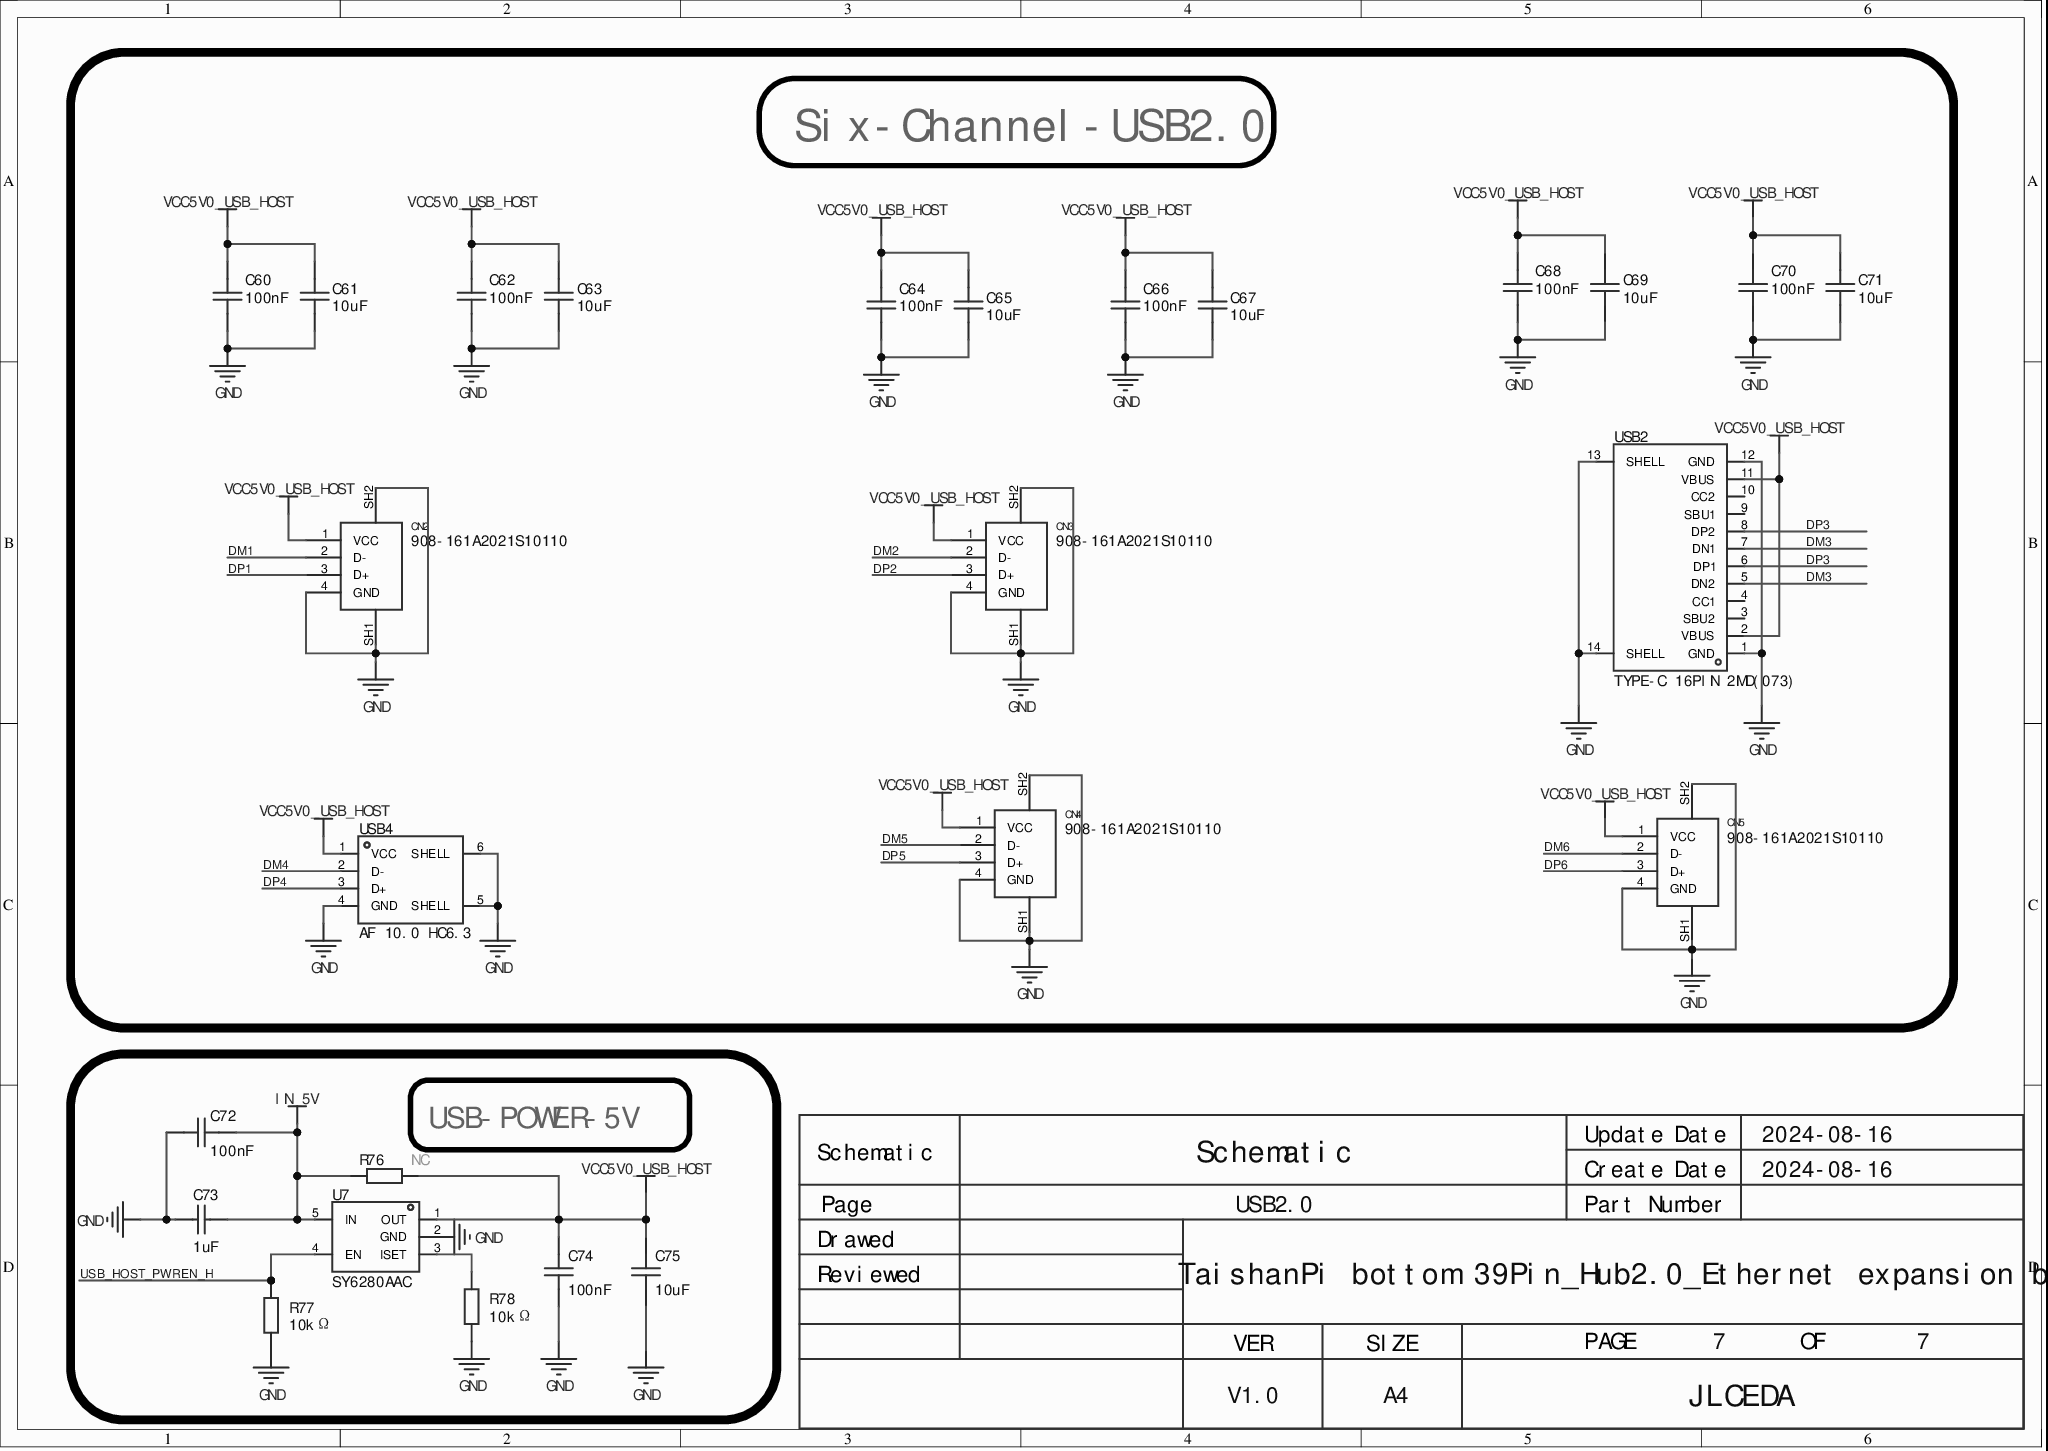
[diagram p0: MISC84334-8.SchDoc]
# Altium project MISC84334.PrjPcb (part 5 of 5)

## Sheet MISC84334-8.SchDoc
size 297 x 210 mm; Symbol: Sheet-Symbol_A4; Company: JLCEDA; Version: V1.0; Page Size: A4; @Project Name: COMPANY_A TaishanPi bottom 39Pin_Hub2.0_Ethernet expansion board; @Page Count: 7; @Update Date: 2024-08-16; @Create Date: 2024-08-16; @Schematic Name: Schematic; @Page No: 7; @Page Name: USB2.0; Device: Sheet-Symbol_A4

### Parts
C60  100nF  [R0402]
C61  10uF  [R0402]
C62  100nF  [r0603]
C63  10uF  [r0603]
C64  100nF  [r0603]
C65  10uF  [r0603]
C66  100nF  [r0603]
C67  10uF  [r0603]
C68  100nF  [r0603]
C69  10uF  [r0603]
C70  100nF  [r0603]
C71  10uF  [r0603]
C72  100nF  [C0603]
C73  1uF  [C0603]
C74  100nF  [C0603]
C75  10uF  [C0603]
CN2  908-161A2021S10110  [USB-A-SMD_AF-SMT-SHORT]
CN3  908-161A2021S10110  [USB-A-SMD_AF-SMT-SHORT]
CN4  908-161A2021S10110  [USB-A-SMD_AF-SMT-SHORT]
CN5  908-161A2021S10110  [USB-A-SMD_AF-SMT-SHORT]
R76  NC  [R0805]
R77  10kΩ  [R0402]
R78  10kΩ  [R0402]
U7  SY6280AAC  [SOT-23-5_L3.0-W1.7-P0.95-LS2.8-BL]
USB2  TYPE-C 16PIN 2MD(073)  [USB-C-SMD_TYPE-C-6PIN-2MD-073]
USB4  AF 10.0 HC6.3  [USB-A-TH_AF-10.0-HC6.3]

### Blocks framed on the sheet
Six-Channel-USB2.0: C60-C71 CN2-CN5 USB2 USB4
USB-POWER-5V: C72-C75 R76-R78 U7

### Nets
GND: C60.1 C61.1 C62.1 C63.1 C64.1 C65.1 C66.1 C67.1 C68.1 C69.1 C70.1 C71.1 C72.2 C73.1 C74.1 C75.1 CN2.4(GND) CN2.SH1 CN2.SH2 CN3.4(GND) CN3.SH1 CN3.SH2 CN4.4(GND) CN4.SH1 CN4.SH2 CN5.4(GND) CN5.SH1 CN5.SH2 R77.1 R78.1 U7.2(GND) USB2.1(GND) USB2.12(GND) USB2.13(SHELL) USB2.14(SHELL) USB4.4(GND) USB4.5(SHELL) USB4.6(SHELL)
IN_5V: C72.1 C73.2 R76.1 U7.5(IN)
VCC5V0_USB_HOST: C60.2 C61.2 C62.2 C63.2 C64.2 C65.2 C66.2 C67.2 C68.2 C69.2 C70.2 C71.2 C74.2 C75.2 CN2.1(VCC) CN3.1(VCC) CN4.1(VCC) CN5.1(VCC) R76.2 U7.1(OUT) USB2.2(VBUS) USB2.11(VBUS) USB4.1(VCC)
DM1: CN2.2(D-)
DM2: CN3.2(D-)
DM3: USB2.5(DN2) USB2.7(DN1)
DM4: USB4.2(D-)
DM5: CN4.2(D-)
DM6: CN5.2(D-)
DP1: CN2.3(D+)
DP2: CN3.3(D+)
DP3: USB2.6(DP1) USB2.8(DP2)
DP4: USB4.3(D+)
DP5: CN4.3(D+)
DP6: CN5.3(D+)
USB_HOST_PWREN_H: R77.2 U7.4(EN)  [project net GPIO0_A5]
NetR78_2: R78.2 U7.3(ISET)

Not connected (* = marked no-connect by the designer): USB2 3(SBU2)* 4(CC1)* 9(SBU1)* 10(CC2)*

### Notes on the sheet
- Update Date
- 2024-08-16
- Schematic
- Page
- USB2.0
- Create Date
- Part Number
- Reviewed
- Drawed
- COMPANY_A TaishanPi bottom 39Pin_Hub2.0_Ethernet expansion board
- VER
- V1.0
- SIZE
- A4
- PAGE
- 7
- JLCEDA
- OF

### Library data of the parts
C60 = CC0402KRX7R7BB104: Capacitance:100nF;Tolerance:±10%;Rated voltage:16V;Dielectric(Temp. coefficient):X7R;; Manufacturer: YAGEO(国巨); Symbol: CC0603KRX7R9BB104; AddInBom: yes; ModelId: 36a51122f27c49738f86b3bfa98863e0; ModelName: C0402_L1.0-W0.5-H0.5; ModelTransform: 39.37,19.685,0,0,0,0,0,0,0; Tolerance: ±10%; Voltage Rated: 16V; Temperature Coefficient: X7R; JLCPCB Part Class: Extended Part; Device: CC0402KRX7R7BB104; LCSC Part Name: 100nF ±10% 16V; SupplierPart: C60474; ManufacturerPart: CC0402KRX7R7BB104; Supplier Footprint: 0402; Datasheet: https://atta.szlcsc.com/upload/public/pdf/source/20211223/9278FD768280B81DDBEF48FA36411A03.pdf; Supplier: LCSC; ConvertToPcb: yes; FootprintName: R0402; Value: 100nF
C61 = CL05A106MQ5NUNC: Capacitance:10uF;Tolerance:±20%;Rated voltage:6.3V;Dielectric(Temp. coefficient):X5R;; Manufacturer: SAMSUNG(三星); Symbol: 0603X106M100; AddInBom: yes; ModelId: 36a51122f27c49738f86b3bfa98863e0; ModelName: C0402_L1.0-W0.5-H0.5; ModelTransform: 39.37,19.685,0,0,0,0,0,0,0; Tolerance: ±20%; Voltage Rated: 6.3V; Temperature Coefficient: X5R; JLCPCB Part Class: Basic Part; Device: CL05A106MQ5NUNC; LCSC Part Name: 10uF ±20% 6.3V; SupplierPart: C15525; ManufacturerPart: CL05A106MQ5NUNC; Supplier Footprint: 0402; Datasheet: https://atta.szlcsc.com/upload/public/pdf/source/20220823/2B02EE04F8F211D38A52DCB16EB6BEBA.pdf; Supplier: LCSC; ConvertToPcb: yes; FootprintName: R0402; Value: 10uF
C62 C64 C66 C68 C70 C72 C74 = CC0603KRX7R9BB104: Capacitance:100nF;Tolerance:±10%;Rated voltage:50V;Dielectric(Temp. coefficient):X7R;; Manufacturer: YAGEO(国巨); AddInBom: yes; ModelId: ac125912035d415993ca9572d50418b1; ModelName: C0603_L1.6-W0.8-H0.8; ModelTransform: 62.992,31.496,0,0,0,0,0,0,0; Tolerance: ±10%; Voltage Rated: 50V; Temperature Coefficient: X7R; Symbol: CC0603KRX7R9BB104; Device: CC0603KRX7R9BB104; LCSC Part Name: 100nF ±10% 50V; SupplierPart: C14663; ManufacturerPart: CC0603KRX7R9BB104; Supplier Footprint: 0603; JLCPCB Part Class: Basic Part; Datasheet: https://atta.szlcsc.com/upload/public/pdf/source/20170116/1484561234239.pdf; Supplier: LCSC; ConvertToPcb: yes; Value: 100nF
  C62 C64 C66 C68 C70: FootprintName: r0603
  C72 C74: FootprintName: C0603
C63 C65 C67 C69 C71 = 0603X106M100CT: Capacitance:10uF;Tolerance:±20%;Rated voltage:10V;Dielectric(Temp. coefficient):X5R;; Manufacturer: Walsin(华新科); AddInBom: yes; ModelId: ac125912035d415993ca9572d50418b1; ModelName: C0603_L1.6-W0.8-H0.8; ModelTransform: 62.992,31.496,0,0,0,0,0,0,0; Tolerance: ±20%; Voltage Rated: 10V; Temperature Coefficient: X5R; Symbol: 0603X106M100; Device: 0603X106M100CT; LCSC Part Name: 10uF ±20% 10V; SupplierPart: C89283; ManufacturerPart: 0603X106M100CT; Supplier Footprint: 0603; JLCPCB Part Class: Extended library; Datasheet: https://atta.szlcsc.com/upload/public/pdf/source/20161226/1482720147964.pdf; Supplier: LCSC; ConvertToPcb: yes; FootprintName: r0603; Value: 10uF
C73 = CL10A105KO8NNNC: Capacitance:1uF;Tolerance:±10%;Rated voltage:16V;Dielectric(Temp. coefficient):X5R;; Manufacturer: SAMSUNG(三星); AddInBom: yes; ModelId: ac125912035d415993ca9572d50418b1; ModelName: C0603_L1.6-W0.8-H0.8; ModelTransform: 62.992,31.496,0,0,0,0,0,0,0; Tolerance: ±10%; Voltage Rated: 16V; Temperature Coefficient: X5R; Symbol: CL10A105KO8NNNC; Device: CL10A105KO8NNNC; LCSC Part Name: 1uF ±10% 16V; SupplierPart: C1592; ManufacturerPart: CL10A105KO8NNNC; Supplier Footprint: 0603; Datasheet: https://atta.szlcsc.com/upload/public/pdf/source/20220919/9FBE606BE0D9532D730F292EB26DC5BB.pdf; Supplier: LCSC; ConvertToPcb: yes; FootprintName: C0603; Value: 1uF
C75 = CL10A106KP8NNNC: Capacitance:10uF;Tolerance:±10%;Rated voltage:10V;Dielectric(Temp. coefficient):X5R;; Manufacturer: SAMSUNG(三星); AddInBom: yes; ModelId: ac125912035d415993ca9572d50418b1; ModelName: C0603_L1.6-W0.8-H0.8; ModelTransform: 62.992,31.496,0,0,0,0,0,0,0; Tolerance: ±10%; Voltage Rated: 10V; Temperature Coefficient: X5R; Symbol: CL10A106KP8NNNC; Device: CL10A106KP8NNNC; LCSC Part Name: 10uF ±10% 10V; SupplierPart: C19702; ManufacturerPart: CL10A106KP8NNNC; Supplier Footprint: 0603; JLCPCB Part Class: Basic Part; Datasheet: https://atta.szlcsc.com/upload/public/pdf/source/20160103/1457707703378.pdf; Supplier: LCSC; ConvertToPcb: yes; FootprintName: C0603; Value: 10uF
CN2-CN5 = 908-161A2021S10110: Connector type:Type-A;Standard:USB 2.0;Gender:Female receptacle;Contacts:4;Ports:1;; Manufacturer: 精拓金; Symbol: USB-CON-AF-SMT-SHORT; AddInBom: yes; ModelId: 83cca92cdad942d3b2896deac7272b6f; ModelName: USB-A-SMD_4P-L14.6-W10.0-H6.3; ModelTransform: 574.802,429.133,0,0,0,0,0,-40.157,-98.425; Connector Type: Type-A; Number of Contacts: 4; Number of Ports: 1; Device: 908-161A2021S10110; Supplier: LCSC; Manufacturer Part: 908-161A2021S10110; Supplier Part: C42595; JLCPCB Part Class: Extended library; LCSC Part Name: Type-A 母座; Supplier Footprint: SMD; ConvertToPcb: yes; FootprintName: USB-A-SMD_AF-SMT-SHORT; Standard: USB 2.0; Gender: Female receptacle
R76 = 0805W8F0000T5E: Resistor type:Thick film resistor;Resistance:0Ω;Tolerance:±1%;Power:125mW;Temp. coefficient:±800ppm/℃;Max working voltage:150V;Operating temperature:-55℃~+155℃;; Manufacturer: UNI-ROYAL(厚声); AddInBom: yes; ModelId: 37a81e68749a4138bd2dfa6897b24b85; ModelName: R0805_L2.0-W1.3-H0.6; ModelTransform: 78.74,51.181,0,0,0,0,0,-0.0005,0; Tolerance: ±1%; Power(Watts): 125mW; Overload Voltage (Max): 150V; Symbol: 0805W8F0000T5E; Value: NC; Device: 0805W8F0000T5E; LCSC Part Name: 0Ω ±1% 125mW; ManufacturerPart: 0805W8F0000T5E; Supplier Footprint: 0805; JLCPCB Part Class: Basic Part; Datasheet: https://atta.szlcsc.com/upload/public/pdf/source/20200306/C422600_1E6D84923E4A46A82E41ADD87F860B5C.pdf; Supplier: LCSC; ConvertToPcb: yes; FootprintName: R0805; Type: Thick film resistor; Temperature Coefficient: ±800ppm/℃; Operating Temperature Range: -55℃~+155℃
R77 R78 = CRCW040210K0FKED: Resistor type:Thick film resistor;Resistance:10kΩ;Tolerance:±1%;Power:63mW;Temp. coefficient:±100ppm/K;Max working voltage:50V;Operating temperature:-55℃~+155℃;; Manufacturer: VISHAY(威世); AddInBom: yes; ModelId: 671aefced39d4c318694bba8bd8efd39; ModelName: R0402_L1.0-W0.5-H0.5; ModelTransform: 39.37,19.685,0,0,0,0,0,0.0005,0; Tolerance: ±1%; Power(Watts): 63mW; Overload Voltage (Max): 50V; Symbol: CRCW040210K0FKED; Device: CRCW040210K0FKED; LCSC Part Name: 10kΩ ±1% 63mW; SupplierPart: C71617; ManufacturerPart: CRCW040210K0FKED; Supplier Footprint: 0402; JLCPCB Part Class: Extended library; Datasheet: https://atta.szlcsc.com/upload/public/pdf/source/20180224/C71617_15194370300791364062.pdf; Supplier: LCSC; ConvertToPcb: yes; FootprintName: R0402; Type: Thick film resistor; Value: 10kΩ; Temperature Coefficient: ±100ppm/K; Operating Temperature Range: -55℃~+155℃
U7 = SY6280AAC_C55136: Low-power power distribution switch; Manufacturer: silergy(矽力杰); AddInBom: yes; ModelId: 0a2a1b8f50944f73965918ad6e5fe167; ModelName: SOT-23-5_L2.9-W1.6-H1.1-LS2.8-P0.95; ModelTransform: 118.60433,114.173,0,90,0,0,0.0005,0.0005,0; Symbol: SY6280AAC; Device: SY6280AAC_C55136; LCSC Part Name: SY6280AAC; SupplierPart: C55136; ManufacturerPart: SY6280AAC; Supplier Footprint: SOT-23-5; JLCPCB Part Class: Extended Part; Datasheet: https://atta.szlcsc.com/upload/public/pdf/source/20161108/1478586372822.pdf; Supplier: LCSC; ConvertToPcb: yes; FootprintName: SOT-23-5_L3.0-W1.7-P0.95-LS2.8-BL
USB2 = TYPE-C 16PIN 2MD(073): Connector type:Type-C;Standard:-;Gender:Female;Contacts:16P;Ports:1;Mounting:Horizontal SMD;Rated current - power:5A;Operating temperature:-25℃~+85℃;; Manufacturer: SHOU HAN(首韩); AddInBom: yes; ModelId: 3a41b9ec9b654a0fad4d118405ec6290; ModelTransform: 351.9678,298.4246,0,0,0,0,0,-47.244,-35.433; Gender: Female; Number of Contacts: 16P; Number of Ports: 1; Current Rating - Power (Max): 5A; Symbol: TYPE-C 16PIN 2MD(073); Device: TYPE-C 16PIN 2MD(073); Supplier: LCSC; Supplier Part: C2765186; Manufacturer Part: TYPE-C 16PIN 2MD(073); LCSC Part Name: Type-C 母 卧贴 带定位柱 不锈钢外壳 2次模顶; Supplier Footprint: SMD; Datasheet: https://atta.szlcsc.com/upload/public/pdf/source/20211123/39B17C16241EAC15C5E277BDA434118E.pdf; ConvertToPcb: yes; FootprintName: USB-C-SMD_TYPE-C-6PIN-2MD-073; ModelName: USB-C-SMD_TYPE-C-6PIN-2MD-073; Connector Type: Type-C; Standard: -; Mounting Style: Horizontal SMD; Operating Temperature Range: -25℃~+85℃
USB4 = AF 10.0 HC6.3: Connector type:Type-A;Standard:USB 2.0;Gender:Female;Ports:1;Contacts:4P;Mounting:Right-angle THT;Rated current - power:1.5A;Operating temperature:-25℃~+85℃;; Manufacturer: SHOU HAN(首韩); AddInBom: yes; ModelId: f9f717efafec4f23bf23d6e98e617557; ModelTransform: 562.991,393.7,0,0,0,0,-0.001,-157.48,-98.425; Connector Type: Type-A; Gender: Female; Number of Ports: 1; Number of Contacts: 4P; Current Rating - Power (Max): 1.5A; Symbol: AF 10.0 HC6.3; Device: AF 10.0 HC6.3; LCSC Part Name: Type-A 母 弯插; SupplierPart: C456017; ManufacturerPart: AF 10.0 HC6.3; Supplier Footprint: 插件; Datasheet: https://atta.szlcsc.com/upload/public/pdf/source/20191113/C456017_24C9995308EDE792CA69BD951BA4C86C.pdf; Supplier: LCSC; ConvertToPcb: yes; FootprintName: USB-A-TH_AF-10.0-HC6.3; ModelName: USB-A-TH_AF-10.0-HC6.3; Standard: USB 2.0; Mounting Style: Right-angle THT; Operating Temperature Range: -25℃~+85℃

## Nets that join several sheets
GND: MISC84334-2 (7 pins), MISC84334-3 (24 pins), MISC84334-4 (37 pins), MISC84334-5 (7 pins), MISC84334-6 (28 pins), MISC84334-7 (28 pins), MISC84334-8 (38 pins)
IN_5V: MISC84334-3 (5 pins), MISC84334-7 (10 pins), MISC84334-8 (C72.1 C73.2 R76.1 U7.5)
VCC1V8: MISC84334-4 (L4.2), MISC84334-6 (6 pins), MISC84334-7 (C13.2 C14.2 U3.5)
VCC3V3_SYS: MISC84334-4 (L5.2 L6.2), MISC84334-5 (R74.2), MISC84334-6 (R71.1), MISC84334-7 (9 pins)
VCC5V0_SYS: MISC84334-2 (FPC1.1 FPC1.2 FPC1.3 FPC1.4), MISC84334-7 (Q1.3 Q2.2)
VCC_4G: MISC84334-6 (11 pins), MISC84334-7 (C4.2 C5.2 R1.2 U1.1)
DM1: MISC84334-3 (U5.18), MISC84334-8 (CN2.2)
DM2: MISC84334-3 (U5.16), MISC84334-8 (CN3.2)
DM3: MISC84334-3 (U5.13), MISC84334-8 (USB2.5 USB2.7)
DM4: MISC84334-3 (U5.11), MISC84334-8 (USB4.2)
DM5: MISC84334-3 (U5.32), MISC84334-8 (CN4.2)
DM6: MISC84334-3 (U5.34), MISC84334-8 (CN5.2)
DMU: MISC84334-2 (FPC1.24), MISC84334-3 (U5.29)
DP1: MISC84334-3 (U5.19), MISC84334-8 (CN2.3)
DP2: MISC84334-3 (U5.17), MISC84334-8 (CN3.3)
DP3: MISC84334-3 (U5.14), MISC84334-8 (USB2.6 USB2.8)
DP4: MISC84334-3 (U5.12), MISC84334-8 (USB4.3)
DP5: MISC84334-3 (U5.33), MISC84334-8 (CN4.3)
DP6: MISC84334-3 (U5.35), MISC84334-8 (CN5.3)
DPU: MISC84334-2 (FPC1.23), MISC84334-3 (U5.30)
GMAC0_INT: MISC84334-2 (FPC1.20), MISC84334-4 (R33.2)
GMAC0_MCLKINOUT: MISC84334-2 (FPC1.19), MISC84334-4 (R28.2)
GMAC0_MDC: MISC84334-2 (FPC1.17), MISC84334-4 (R21.2 U4.13)
GMAC0_MDIO: MISC84334-2 (FPC1.18), MISC84334-4 (R20.2 U4.14)
GMAC0_RSTN: MISC84334-2 (FPC1.21), MISC84334-4 (C22.2 R42.1 U4.12)
GMAC0_RXCLK: MISC84334-2 (FPC1.10), MISC84334-4 (R26.2 R41.2)
GMAC0_RXD0: MISC84334-2 (FPC1.14), MISC84334-4 (R13.2 R44.2)
GMAC0_RXD1: MISC84334-2 (FPC1.15), MISC84334-4 (R16.2 R45.2)
GMAC0_RXD2: MISC84334-2 (FPC1.8), MISC84334-4 (R22.2 R46.2)
GMAC0_RXD3: MISC84334-2 (FPC1.9), MISC84334-4 (R18.2 R48.2)
GMAC0_RXDV_CRS: MISC84334-2 (FPC1.16), MISC84334-4 (R30.2 R43.2)
GMAC0_TXCLK: MISC84334-2 (FPC1.7), MISC84334-4 (U4.20)
GMAC0_TXD0: MISC84334-2 (FPC1.11), MISC84334-4 (U4.18)
GMAC0_TXD1: MISC84334-2 (FPC1.12), MISC84334-4 (U4.17)
GMAC0_TXD2: MISC84334-2 (FPC1.5), MISC84334-4 (U4.16)
GMAC0_TXD3: MISC84334-2 (FPC1.6), MISC84334-4 (U4.15)
GMAC0_TXEN: MISC84334-2 (FPC1.13), MISC84334-4 (U4.19)
GPIO0_A5: MISC84334-2 (FPC1.38), MISC84334-8 (R77.2 U7.4)
GPIO0_C5: MISC84334-2 (FPC1.39), MISC84334-5 (C59.1 R74.1 R75.1)
HP_SNS: MISC84334-2 (FPC1.33), MISC84334-5 (AUDIO1.2 R73.1)
HPL_OUT: MISC84334-2 (FPC1.32), MISC84334-5 (AUDIO1.4)
HPR_OUT: MISC84334-2 (FPC1.34), MISC84334-5 (AUDIO1.3)
HUB_DM7: MISC84334-3 (U5.37), MISC84334-6 (R68.2)
HUB_DP7: MISC84334-3 (U5.38), MISC84334-6 (R69.2)
PCIE_TS_RX: MISC84334-2 (FPC1.36), MISC84334-6 (Q5.3 R71.2)
PCIE_TS_TX: MISC84334-2 (FPC1.37), MISC84334-6 (Q4.2)